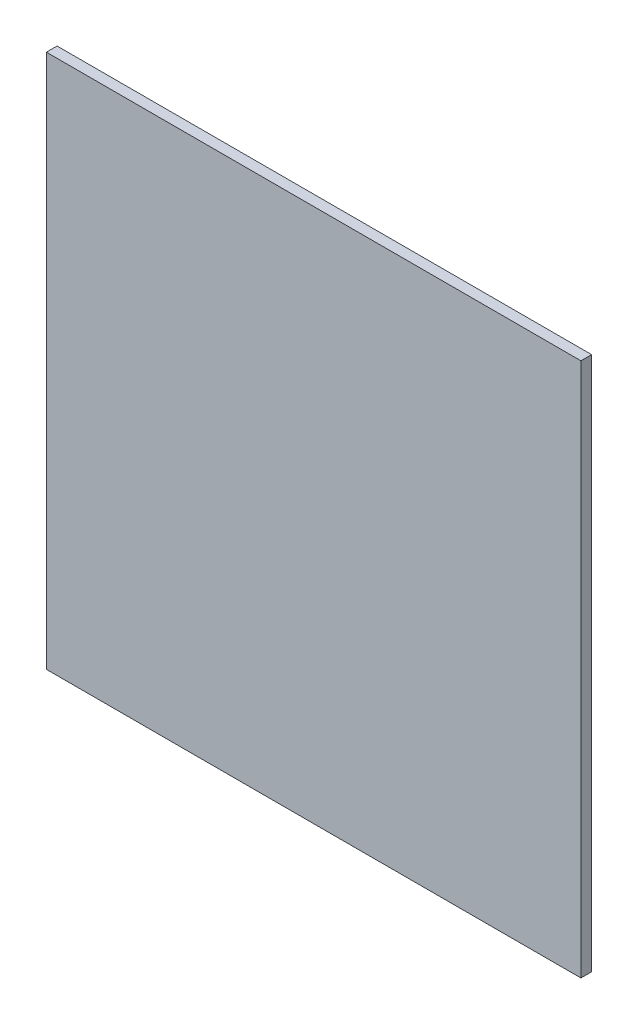
from build123d import *

# Parameters (mm, degrees)
SKETCH1_W           = 50
SKETCH1_H           = 50
BOSS_EXTRUDE1_DEPTH = 1


with BuildPart() as part:
    # Sketch1 → Boss-Extrude1 (new body)
    with BuildSketch(Plane.XY):
        Rectangle(SKETCH1_W, SKETCH1_H)
    extrude(amount=BOSS_EXTRUDE1_DEPTH)


solid = part.part
